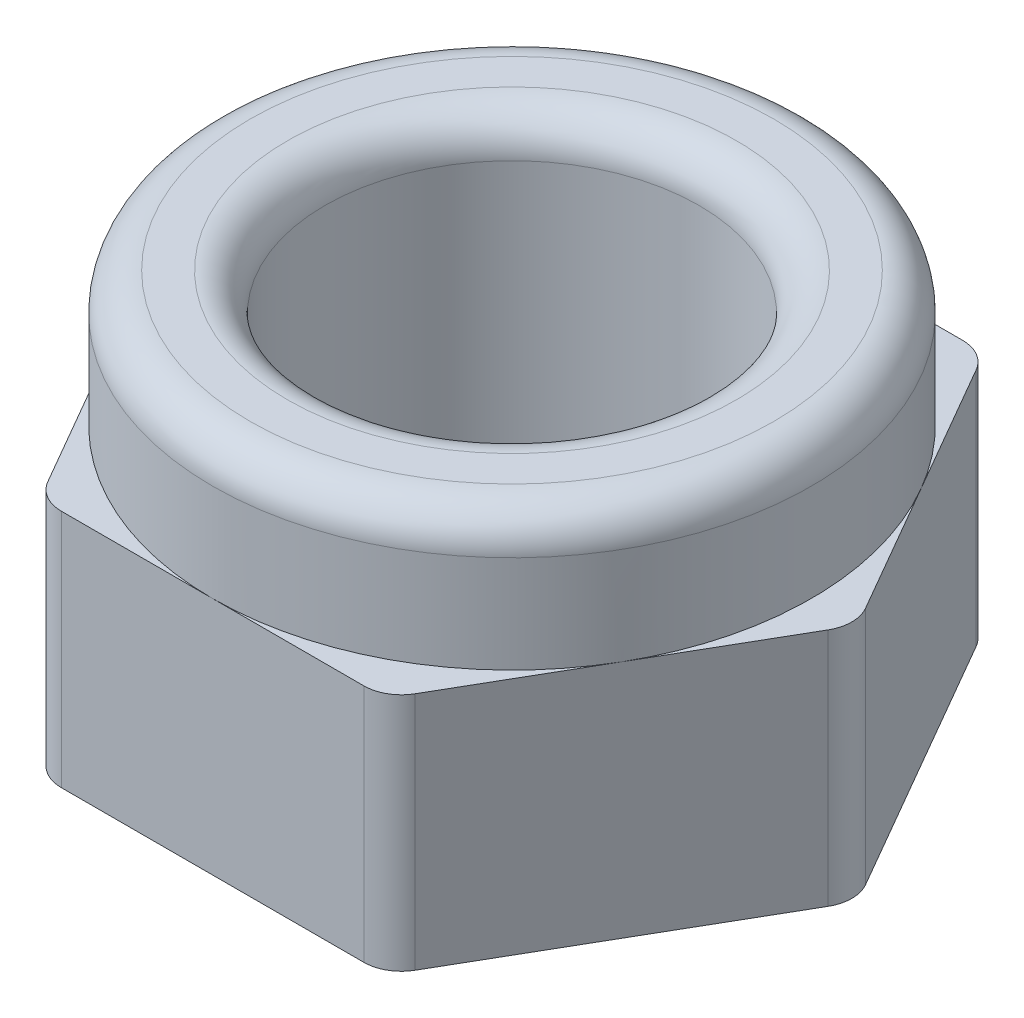
SolidWorks part; units mm, degrees
material "AISI 304"
ref_plane "前视基准面" through (0, 0, 0) normal (0, 0, 1) x (1, 0, 0)
ref_plane "上视基准面" through (0, 0, 0) normal (0, 1, 0) x (1, 0, 0)
ref_plane "右视基准面" through (0, 0, 0) normal (1, 0, 0) x (0, 0, -1)
sketch "草图1" plane through (0, 0, 0) normal (0, 1, 0) x (1, 0, 0)
  line L1 (4.6188, 0) -> (2.3094, 4)
  line L2 (2.3094, 4) -> (-2.3094, 4)
  line L3 (-2.3094, 4) -> (-4.6188, 0)
  line L4 (-4.6188, 0) -> (-2.3094, -4)
  line L5 (-2.3094, -4) -> (2.3094, -4)
  line L6 (2.3094, -4) -> (4.6188, 0)
  circle A0 centre (0, 0) radius 4 construction
  circle A1 centre (0, 0) radius 2.5
  dimension "D2" = 5
  dimension "D1" = 8
extrude "凸台-拉伸1" add sketch "草图1" along normal blind 3.2
sketch "草图2" plane through (0, 3.2, 0) normal (0, 1, 0) x (1, 0, 0)
  line L0 (-4.6188, 0) -> (-2.3094, -4) construction
  circle A0 centre (0, 0) radius 4
  circle A1 centre (0, 0) radius 2.5 construction
  circle A2 centre (0, 0) radius 2.5
extrude "凸台-拉伸2" add sketch "草图2" along normal blind 1.8
fillet "圆角3" radius 0.5 8 edges at (0, 5, 2.5) (0, 5, 4) (-4.6188, 1.6, 0) (-2.3094, 1.6, 4) (-2.3094, 1.6, -4) (2.3094, 1.6, -4) (4.6188, 1.6, 0) (2.3094, 1.6, 4)
